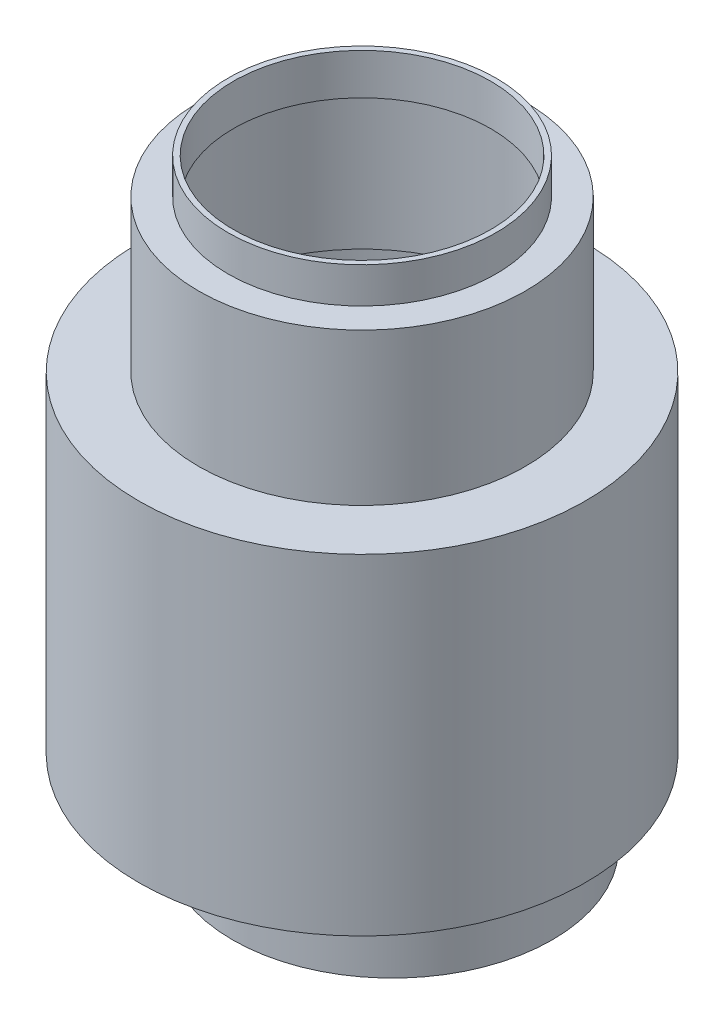
SolidWorks part; units mm, degrees
ref_plane "Front plane" through (0, 0, 0) normal (0, 0, 1) x (1, 0, 0)
ref_plane "Top plane" through (0, 0, 0) normal (0, 1, 0) x (1, 0, 0)
ref_plane "Right plane" through (0, 0, 0) normal (1, 0, 0) x (0, 0, -1)
sketch "Sketch1" plane through (0, 0, 0) normal (0, 0, 1) x (1, 0, 0)
  line L0 (0, 0) -> (125, 0)
  line L1 (125, 0) -> (125, 185)
  line L2 (125, 185) -> (91.5, 185)
  line L3 (91.5, 185) -> (91.5, 270)
  line L4 (91.5, 270) -> (75, 270)
  line L5 (75, 270) -> (75, 290)
  line L6 (75, 290) -> (0, 290)
  line L7 (0, 290) -> (0, 0)
  point P4 (83.25, 270)
  point P10 (91.5, 227.5)
  dimension "D1" = 75
  dimension "D2" = 20
  dimension "D3" = 91.5
  dimension "D4" = 85
  dimension "D5" = 185
  dimension "D6" = 125
revolve "Revolve1" add sketch "Sketch1" angle 360 about L7
sketch "Sketch2" plane through (0, 0, 0) normal (0, -1, 0) x (1, 0, 0)
  circle A0 centre (17, 0) radius 89.5
  dimension "D1" = 179
  dimension "D2" = 17
extrude "Boss-Extrude1" add sketch "Sketch2" along normal blind 37
shell "Shell1" thickness 3
